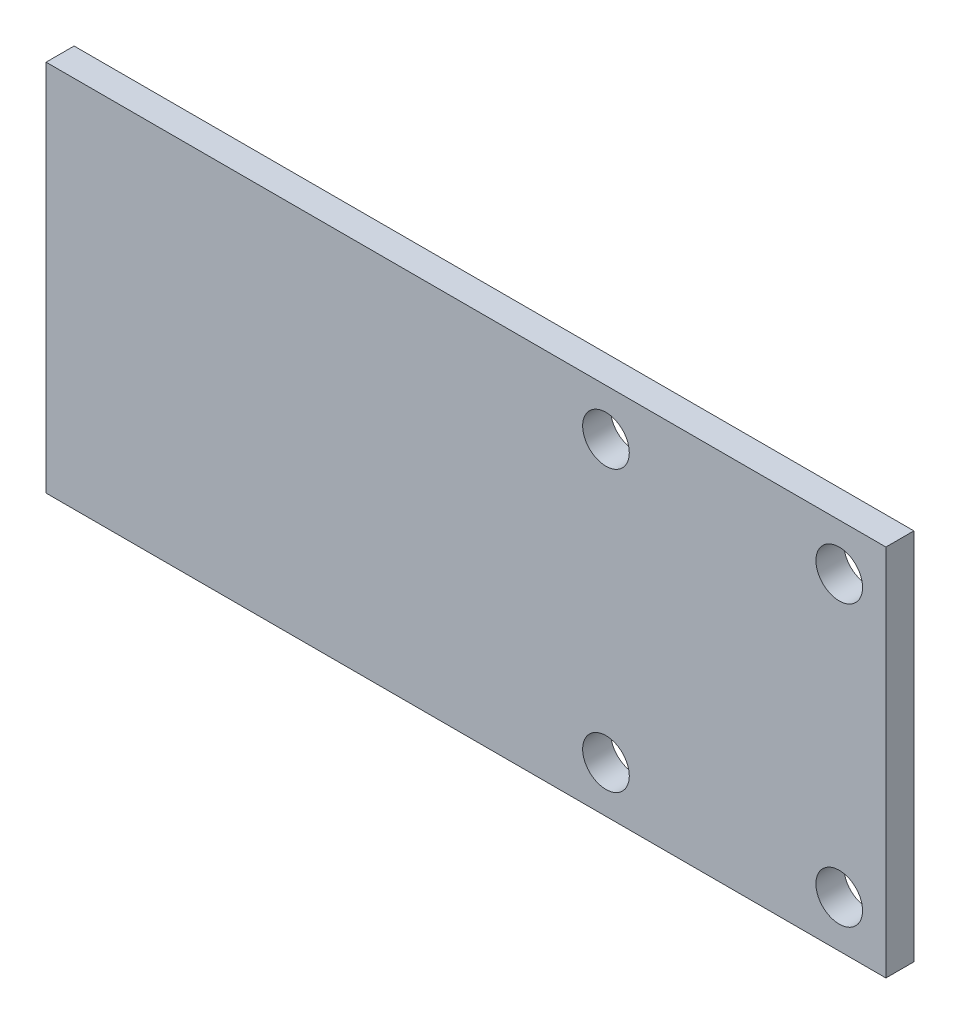
from build123d import *

# Parameters (mm, degrees)
SKETCH_1_W          = 180
SKETCH_1_H          = 80
EXTRUDE_1_DEPTH     = 6
SKETCH_2_R          = 5
CUT_EXTRUDE_1_DEPTH = 6


with BuildPart() as part:
    # 草图1 → 凸台-拉伸1 (new body)
    with BuildSketch(Plane.XY):
        with Locations((90, 40)):
            Rectangle(SKETCH_1_W, SKETCH_1_H)
    extrude(amount=EXTRUDE_1_DEPTH)

    # 草图2 → 切除-拉伸1 (cut)
    with BuildSketch(Plane.XY.offset(6)):
        with Locations((170, 69.998664645)):
            Circle(SKETCH_2_R)
        with Locations((120, 9.998664645)):
            Circle(SKETCH_2_R)
        with Locations((120, 69.998664645)):
            Circle(SKETCH_2_R)
        with Locations((170, 9.998664645)):
            Circle(SKETCH_2_R)
    extrude(amount=-CUT_EXTRUDE_1_DEPTH, mode=Mode.SUBTRACT)


solid = part.part
